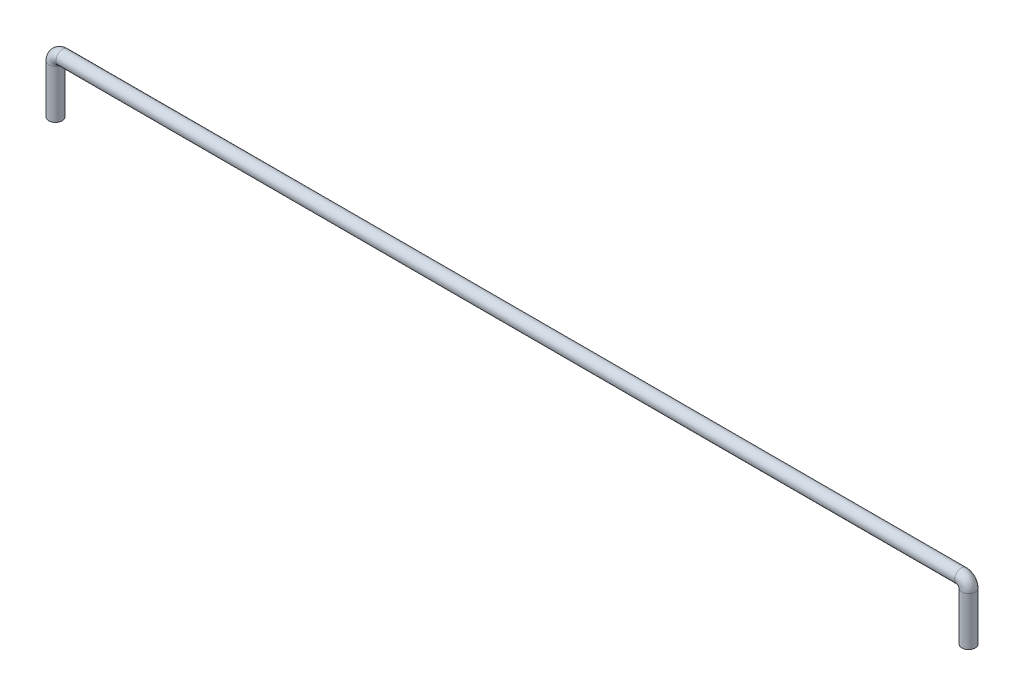
SolidWorks part; units mm, degrees
ref_plane "Front Plane" through (0, 0, 0) normal (0, 0, 1) x (1, 0, 0)
ref_plane "Top Plane" through (0, 0, 0) normal (0, 1, 0) x (1, 0, 0)
ref_plane "Right Plane" through (0, 0, 0) normal (1, 0, 0) x (0, 0, -1)
sketch "Sketch1" plane through (0, 0, 0) normal (0, 0, 1) x (1, 0, 0)
  line L0 (-49.2377, -16.8593) -> (-49.2377, 26.6407)
  line L1 (-42.7377, 33.1407) -> (763.2623, 33.1407)
  line L2 (769.7623, 26.6407) -> (769.7623, -16.8593)
  arc A0 (769.7623, 26.6407) -> (763.2623, 33.1407) centre (763.2623, 26.6407) ccw
  arc A1 (-42.7377, 33.1407) -> (-49.2377, 26.6407) centre (-42.7377, 26.6407) ccw
  point P6 (769.7623, 33.1407)
  point P9 (-49.2377, 33.1407)
  dimension "D4" = 6.5
  dimension "D1" = 50
  dimension "D2" = 50
  dimension "D3" = 819
  dimension "D5" = 90
  dimension "D6" = 90
ref_plane "Plane1" through (-49.2377, -16.8593, 0) normal (0, 1, 0) x (-1, 0, 0)
sketch "Sketch2" plane through (-49.2377, -16.8593, 0) normal (0, 1, 0) x (-1, 0, 0)
  circle A0 centre (0, 0) radius 6
sweep "Sweep1" add profiles "Sketch2" path "Sketch1"
